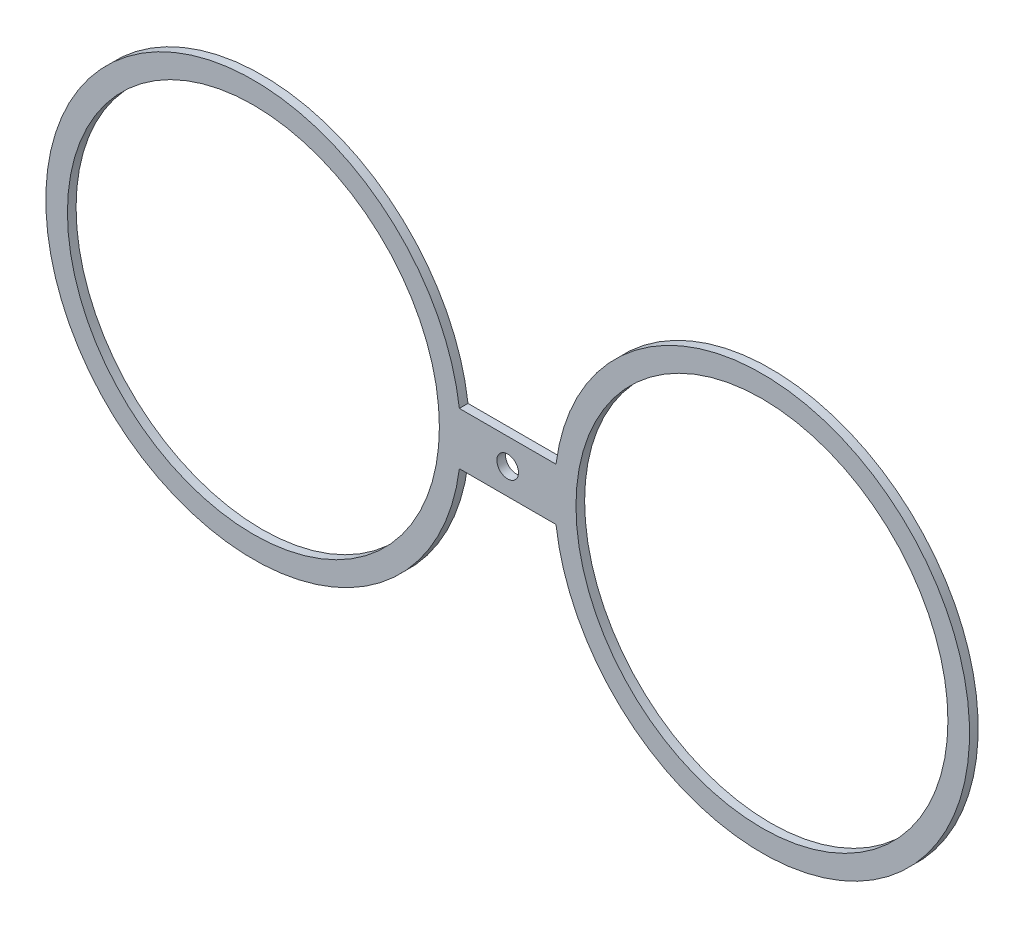
from build123d import *

# Parameters (mm, degrees)
SKETCH1_R           = 43
SKETCH1_R_2         = 2.5
BOSS_EXTRUDE1_DEPTH = 2


with BuildPart() as part:
    # Sketch1 → Boss-Extrude1 (new body)
    with BuildSketch(Plane.XY):
        with BuildLine():
            Line((47.617811618, 6.045164742), (69.962188382, 6.045164742))
            ThreePointArc((69.962188382, 6.045164742), (165.579998377, -0.012483332), (69.959050499, -6.020396052))
            Line((69.959050499, -6.020396052), (47.620949501, -6.020396052))
            ThreePointArc((47.620949501, -6.020396052), (-47.999998377, -0.012483332), (47.617811618, 6.045164742))
        make_face()
        Circle(SKETCH1_R, mode=Mode.SUBTRACT)
        with Locations((117.58, 0)):
            Circle(SKETCH1_R, mode=Mode.SUBTRACT)
        with Locations((58.79, 0)):
            Circle(SKETCH1_R_2, mode=Mode.SUBTRACT)
    extrude(amount=BOSS_EXTRUDE1_DEPTH)


solid = part.part
